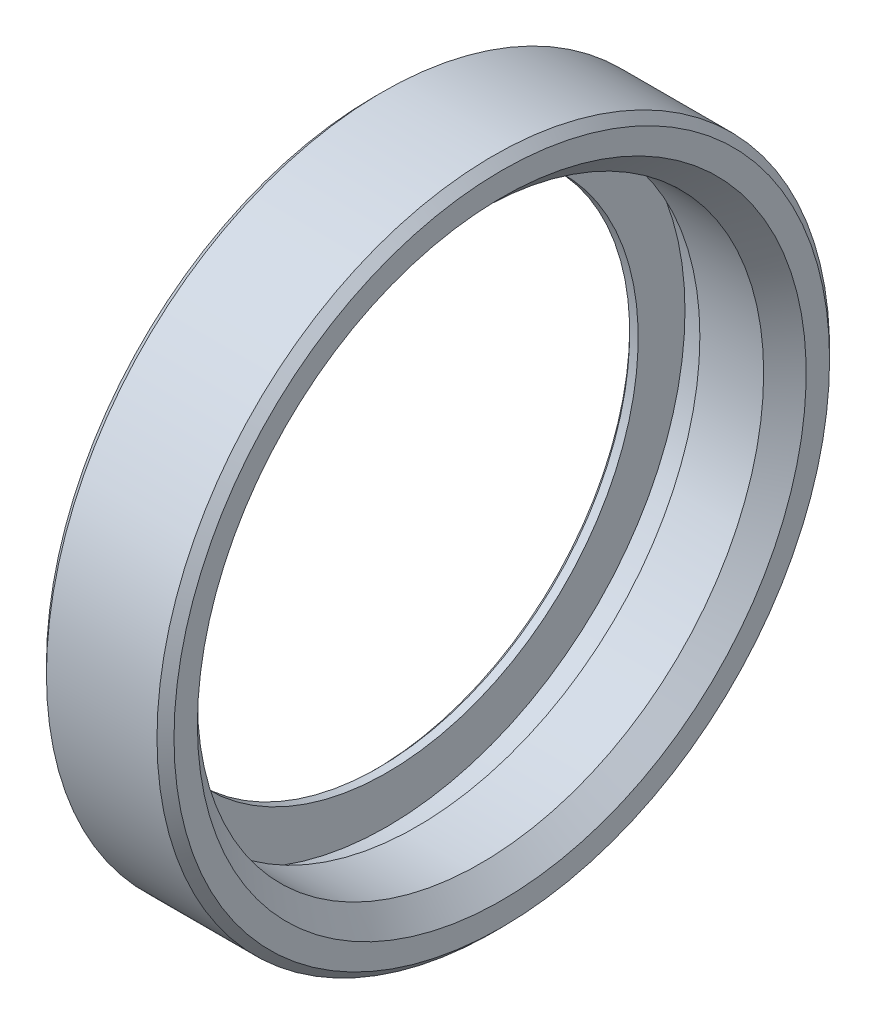
SolidWorks part; units mm, degrees
material "A6061"
ref_plane "Front Plane" through (0, 0, 0) normal (0, 0, 1) x (1, 0, 0)
ref_plane "Top Plane" through (0, 0, 0) normal (0, 1, 0) x (1, 0, 0)
ref_plane "Right Plane" through (0, 0, 0) normal (1, 0, 0) x (0, 0, -1)
sketch "Sketch1" plane through (0, 0, 0) normal (0, 0, 1) x (1, 0, 0)
  line L0 (1539.3526, 1902.8732) -> (1552.7977, 1902.8732) construction
  line L13 (1541.966, 1896.1493) -> (1541.8522, 1896.0355)
  line L14 (1541.966, 1896.1493) -> (1542.1936, 1896.1493)
  line L15 (1541.8522, 1894.1008) -> (1542.0798, 1893.8732)
  line L16 (1541.8522, 1896.0355) -> (1541.8522, 1894.1008)
  line L17 (1542.1936, 1896.1493) -> (1542.1936, 1894.8974)
  line L18 (1544.6974, 1895.2958) -> (1542.9903, 1895.2958)
  line L19 (1544.9819, 1895.0112) -> (1542.9903, 1895.0112)
  line L20 (1542.1936, 1894.8974) -> (1542.9903, 1894.8974)
  line L21 (1542.9903, 1895.2958) -> (1542.9903, 1894.8974)
  line L22 (1545.2664, 1894.7267) -> (1544.6974, 1895.2958)
  line L23 (1545.2664, 1894.7267) -> (1545.2664, 1894.1008)
  line L24 (1542.0798, 1893.8732) -> (1545.0388, 1893.8732)
  line L25 (1545.2664, 1894.1008) -> (1545.0388, 1893.8732)
  dimension "D1" = 9
revolve "Revolve1" add sketch "Sketch1" angle 360 about L0
equation "\"a\"= \"名称代码\""
equation "\"b\"= \"图号代码\""
